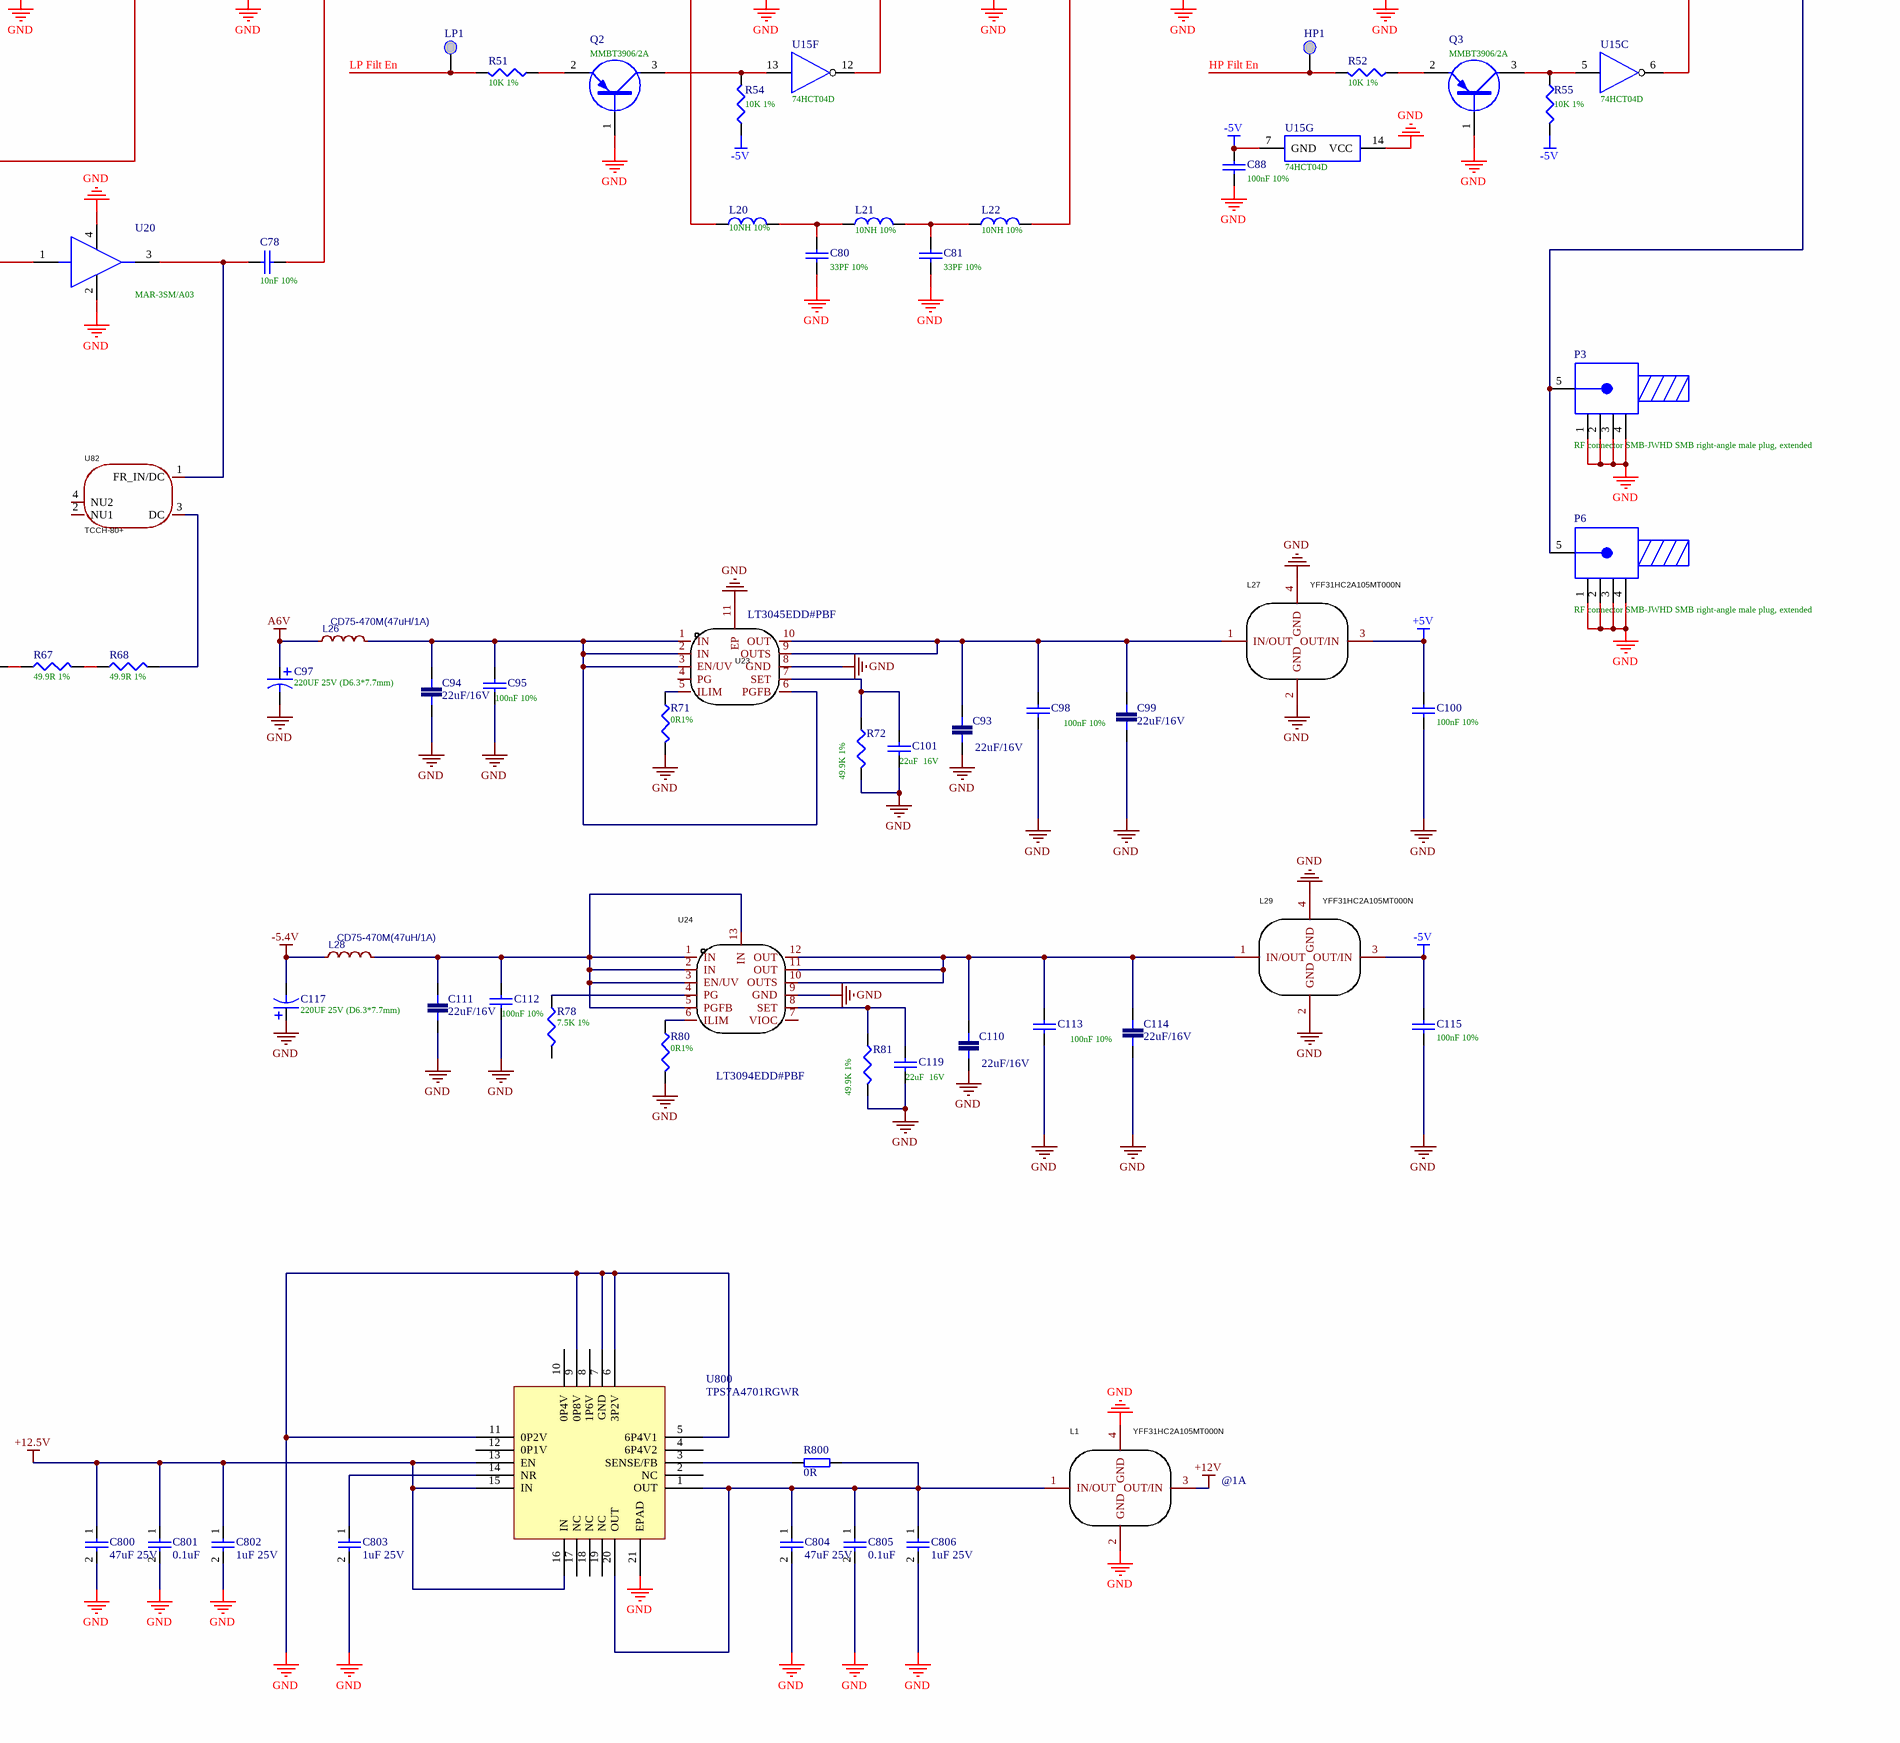
[diagram p0: PCBE109560-10.SchDoc, bottom right]
# Altium schematic sheet PCBE109560-10.SchDoc (part 2 of 2)

## Parts
1  (no value)  [DIP-1]
+1  (no value)  [DIP-1]
+2  (no value)  [DIP-1]
C4  20PF 10%  [0805C]
C5  330PF 10%  [1812C]
C6  22PF 10%  [1812C-2]
C7  22uF/16V  [0805]
C8  22uF/16V  [0805]
C9  100nF 10%  [0603]
C10  220UF 25V (D6.3*7.7mm)  [CAP-SMD_BD6.3-L6.6-W6.6-FD]
C11  100nF 10%  [0603]
C12  22uF/16V  [0805]
C13  100nF 10%  [0805R]
C14  22uF  16V  [0805]
C15  100nF 10%  [0805R]
C16  47PF 10%  [1812C-2]
C17  100PF 10%  [1812C-2]
C18  20PF 10%  [0805R]
C20  100nF 10%  [0805R]
C21  100nF 10%  [0805R]
C31  100nF 10%  [0805R]
C32  100nF 10%  [0805R]
C34  100nF 10%  [0805R]
C35  100nF 10%  [0805R]
C36  100nF 10%  [0805R]
C37  100nF 10%  [0805R]
C39  100nF 10%  [0805R]
C40  100nF 10%  [0805R]
C41  100nF 10%  [0805R]
C42  100nF 10%  [0805R]
C43  100nF 10%  [0805R]
C44  100nF 10%  [0805R]
C45  100nF 10%  [0805R]
C46  100nF 10%  [0805R]
C47  100nF 10%  [0805R]
C48  100nF 10%  [0805R]
C49  22uF 25V  [CAP-SMD_L6.0-W3.2-R-RD]
C50  100nF 10%  [0805R]
C51  100nF 10%  [0805R]
C52  100nF 10%  [0805R]
C53  3.3NF 10%  [0805R]
C54  100nF 10%  [0805R]
C55  330PF 10%  [0805R]
C56  330PF 10%  [0805R]
C57  100nF 10%  [0805R]
C58  33PF 10%  [0805R]
C59  33PF 10%  [0805R]
C60  100nF 10%  [0805R]
C61  100nF 10%  [0805R]
C62  100nF 10%  [0805R]
C63  100nF 10%  [0805R]
C64  100nF 10%  [0805R]
C65  33PF 10%  [0805R]
C66  33PF 10%  [0805R]
C67  100nF 10%  [0805R]
C68  39PF 10%  [0805R]
C69  100nF 10%  [0805R]
C70  25V 1UF Type A  [0805C-2]
C71  25V 1UF Type A  [0805C-2]
C72  100nF 10%  [0805R]
C73  25V 1UF Type A  [0805C-2]
C74  100nF 10%  [0805R]
C75  100nF 10%  [0805R]
C76  10nF 10%  [0805R]
C77  10nF 10%  [0805R]
C78  10nF 10%  [0805R]
C79  100nF 10%  [0603C]
C80  33PF 10%  [0805R]
C81  33PF 10%  [0805R]
C82  100nF 10%  [0805R]
C83  100nF 10%  [0805R]
C84  100nF 10%  [0805R]
C85  100nF 10%  [0805R]
C86  25V 1UF Type A  [0805C-2]
C87  3pF( ±0.1pF)  [0805R]
C88  100nF 10%  [0805R]
C89  100nF 10%  [0805R]
C90  100nF 10%  [0805R]
C93  22uF/16V  [0805]
C94  22uF/16V  [0805]
C95  100nF 10%  [0603]
C96  100nF 10%  [0805R]
C97  220UF 25V (D6.3*7.7mm)  [CAP-SMD_BD6.3-L6.6-W6.6-FD]
C98  100nF 10%  [0603]
C99  22uF/16V  [0805]
C100  100nF 10%  [0805R]
C101  22uF  16V  [0805]
C102  100nF 10%  [0805R]
C103  100nF 10%  [0805R]
C104  100nF 10%  [0805R]
C105  100nF 10%  [0805R]
C106  100nF 10%  [0805R]
C107  100nF 10%  [0805R]
C109  100nF 10%  [0805R]
C110  22uF/16V  [0805]
C111  22uF/16V  [0805]
C112  100nF 10%  [0603]
C113  100nF 10%  [0603]
C114  22uF/16V  [0805]
C115  100nF 10%  [0805R]
C116  100nF 10%  [0805R]
C117  220UF 25V (D6.3*7.7mm)  [CAP-SMD_BD6.3-L6.6-W6.6-FD]
C118  100nF 10%  [0805R]
C119  22uF  16V  [0805]
C122  100nF 10%  [0805R]
C123  100nF 10%  [0805R]
C124  100nF 10%  [0805R]
C125  100nF 10%  [0805R]
C128  100nF 10%  [0805R]
C129  100nF 10%  [0805R]
C130  100nF 10%  [0805R]
C800  47uF 25V  [1206]
C801  0.1uF  [0402]
C802  1uF 25V  [0402]
C803  1uF 25V  [0402]
C804  47uF 25V  [1206]
C805  0.1uF  [0402]
C806  1uF 25V  [0402]
C888  100nF 10%  [0805R]
Clk1  (no value)  [DIP-1]
D1  BAV99/A7  [SOT-23]
D2  GF1M-E3/67A/GM  [1808D]
D3  GF1M-E3/67A/GM  [1808D]
D4  GF1M-E3/67A/GM  [1808D]
D5  GF1M-E3/67A/GM  [1808D]
D8  BAV99/A7  [SOT-23-2]
D9  BAV99/A7  [SOT-23-2]
D10  BAV99/A7  [SOT-23-2]
D11  BAV99/A7  [SOT-23-2]
D12  BAV99/A7  [SOT-23-2]
Data1  (no value)  [DIP-1]
HP1  (no value)  [DIP-1]
J1  RF connector  [DIP-P]
J2  RF connector  [DIP-P]
L1  YFF31HC2A105MT000N  [FILTER-SMD_4P-L3.2-W1.6-L_YFF31HC]
L2  15UH 5%  [1005R]
L3  BLM21PG221SN1D(220Ω@100MHz)  [0805R]
L4  YFF31HC2A105MT000N  [FILTER-SMD_4P-L3.2-W1.6-L_YFF31HC]
L5  6.8UH 10%  [0805R]
L8  YFF31HC2A105MT000N  [FILTER-SMD_4P-L3.2-W1.6-L_YFF31HC]
L10  10NH 10%  [0805R]
L11  10NH 10%  [0805R]
L12  10NH 10%  [0805R]
L13  YFF31HC2A105MT000N  [FILTER-SMD_4P-L3.2-W1.6-L_YFF31HC]
L15  4.7UH 5%  [1005L]
L16  1UH 5%  [0805R]
L17  BLM21PG221SN1D(220Ω@100MHz)  [0805R]
L18  BLM21PG221SN1D(220Ω@100MHz  [0805R]
L19  NFM15PC104R1A3D  [FILTER-SMD_0402-3P-L1.0-W0.5-T]
L20  10NH 10%  [0805R]
L21  10NH 10%  [0805R]
L22  10NH 10%  [0805R]
L23  YFF31HC2A105MT000N  [FILTER-SMD_4P-L3.2-W1.6-L_YFF31HC]
L24  YFF31HC2A105MT000N  [FILTER-SMD_4P-L3.2-W1.6-L_YFF31HC]
L25  BLM21PG221SN1D(220Ω@100MHz  [0805R]
L26  CD75-470M(47uH/1A)  [IND-SMD_L7.8-W7.0-A]
L27  YFF31HC2A105MT000N  [FILTER-SMD_4P-L3.2-W1.6-L_YFF31HC]
L28  CD75-470M(47uH/1A)  [IND-SMD_L7.8-W7.0-A]
L29  YFF31HC2A105MT000N  [FILTER-SMD_4P-L3.2-W1.6-L_YFF31HC]
L31  BLM21PG221SN1D(220Ω@100MHz  [0805R]
L32  BLM21PG221SN1D(220Ω@100MHz  [0805R]
L808  NFM15PC104R1A3D  [FILTER-SMD_0402-3P-L1.0-W0.5-T]
L809  NFM15PC104R1A3D  [FILTER-SMD_0402-3P-L1.0-W0.5-T]
L810  NFM15PC104R1A3D  [FILTER-SMD_0402-3P-L1.0-W0.5-T]
L811  NFM15PC104R1A3D  [FILTER-SMD_0402-3P-L1.0-W0.5-T]
L812  NFM15PC104R1A3D  [FILTER-SMD_0402-3P-L1.0-W0.5-T]
L813  NFM15PC104R1A3D  [FILTER-SMD_0402-3P-L1.0-W0.5-T]
LP1  (no value)  [DIP-1]
P1  Header 20X2  [N0.8mm/40Pin-Plug]
P2  Header 4X2  [N0.8mm/8Pin-SOCKET]
P3  RF connector SMB-JWHD SMB right-angle male plug, extended  [DIP-P-2]
P4  Header 20X2  [N0.8mm/40Pin-Plug]
P5  Header 20X2  [N0.8mm/40Pin-Plug]
P6  RF connector SMB-JWHD SMB right-angle male plug, extended  [DIP-P-2]
Q1  MJD31C  [SOT-252-2]
Q2  MMBT3906/2A  [SOT-23]
Q3  MMBT3906/2A  [SOT-23]
Q4  MMBT3906/2A  [SOT-23]
R6  2K 5%  [0603R]
R7  NC  [AXIAL-0.51]
R8  3.9K 5% 1/2W  [AXIAL-0.51]
R9  3.9K 5% 1/2W  [AXIAL-0.51]
R10  3.9K 5% 1/2W  [AXIAL-0.51]
R11  3.9K 5% 1/2W  [AXIAL-0.51]
R13  0R1%  [0603]
R14  49.9K 1%  [0603]
R15  4.99K 1%  [0805R]
R16  2K 1%  [0805R]
R17  49.9R 1% 1/4W  [AXIAL-0.4]
R20  100R 1% 1/4W  [AXIAL-0.4]
R23  100R 1% 1/4W  [AXIAL-0.4]
R27  4.87K 1%  [0805R]
R28  4.87K 1%  [0805R]
R29  4.87K 1%  [0805R]
R30  4.87K 1%  [0805R]
R31  4.87K 1%  [0805R]
R32  10K 1%  [0805R]
R33  100K 1%  [0805R]
R34  100K 1%  [0805R]
R35  49.9R 1%  [0805R]
R36  49.9R 1%  [0805R]
R37  49.9R 1%  [0805R]
R38  49.9R 1%  [0805R]
R39  49.9R 1%  [0805R]
R40  49.9R 1% 1/4W  [R-SMD_L3.5-W1.5]
R41  10K 1%  [0805R]
R42  4.87K 1%  [0805R]
R43  4.87K 1%  [0805R]
R44  4.87K 1%  [0805R]
R45  4.87K 1%  [0805R]
R46  169R 1%  [0805R]
R47  169R 1%  [0805R]
R48  169R 1%  [0805R]
R49  49.9R 1%  [0805R]
R50  49.9R 1%  [0805R]
R51  10K 1%  [0805R]
R52  10K 1%  [0805R]
R53  10K 1%  [0805R]
R54  10K 1%  [0805R]
R55  10K 1%  [0805R]
R56  10K 1%  [0805R]
R57  10K 1%  [0805R]
R58  49.9R 1%  [0805R]
R59  4.99K 1%  [0805R]
R60  49.9R 1%  [R-SMD_L3.5-W1.5]
R61  30R 1%  [R-SMD_L3.5-W1.5]
R62  169R 1%  [0805R]
R63  169R 1%  [0805R]
R64  169R 1%  [0805R]
R65  49.9R 1%  [0805R]
R66  49.9R 1%  [0805R]
R67  49.9R 1%  [0805R]
R68  49.9R 1%  [0805R]
R69  120R 1%  [R-SMD_L3.5-W1.5]
R70  169R 1%  [0805R]
R71  0R1%  [0603]
R72  49.9K 1%  [0603]
R73  169R 1%  [0805R]
R74  NC  [0805R]
R75  169R 1%  [0805R]
R77  169R 1%  [0805R]
R78  7.5K 1%  [0603]
R80  0R1%  [0603]
R81  49.9K 1%  [0603]
R82  100K 1%  [0805R]
R83  10K 1%  [0805R]
R84  169R 1%  [0805R]
R800  0R  [0402]
RE1  AGQ210A4HZ  [RELAY-SMD_PANASONIC_AGQ2X0AXX]
RE2  AGQ210A4HZ  [RELAY-SMD_PANASONIC_AGQ2X0AXX]
RE3  AGQ210A4HZ  [RELAY-SMD_PANASONIC_AGQ2X0AXX]
RE4  AGQ210A4HZ  [RELAY-SMD_PANASONIC_AGQ2X0AXX]
RE5  AGQ210A4HZ  [RELAY-SMD_PANASONIC_AGQ2X0AXX]
Strobe1  (no value)  [DIP-1]
U4  LT3045EDD#PBF  [DFN-10_L3.0-W3.0-P0.50-BL-EP]
U6  74HCT123D  [SOIC-16_L9.9-W3.9-P1.27-LS6.0-BL]
U8  MAX504CSD+T  [SO-14]
U9  SW-239  [SO-8]
U11  SW-239  [SO-8]
U12  SW-239  [SO-8]
U13  SW-239  [SO-8]
U14  SW-239  [SO-8]
U15  74HCT04D  [SO-14]  (parts A,B,C,D,E,F,G of 7)
U16  AT-250(MAAV-007941)  [SO-8]
U17  MAR-3SM/A03  [LCC4]
U18  MAR-6SM/A06  [LCC4]
U19  MAR-6SM/A06  [LCC4]
U20  MAR-3SM/A03  [LCC4]
U21  MAX4106ESA+T  [SO-8]
U22  MIC4420CM  [SO-8]
U23  LT3045EDD#PBF  [DFN-10_L3.0-W3.0-P0.50-BL-EP]
U24  LT3094EDD#PBF  [WDFN-12_L3.0-W3.0-P0.45-BL-EP]
U25  AT65-0263  [SO-16]
U80  TCCH-80+  [IND-SMD_4P-L3.8-W3.8]
U81  TCCH-80+  [IND-SMD_4P-L3.8-W3.8]
U82  TCCH-80+  [IND-SMD_4P-L3.8-W3.8]
U83  TCCH-80+  [IND-SMD_4P-L3.8-W3.8]
U100  SW-239  [SO-8]
U800  TPS7A4701RGWR  [QFN-20]

## Nets
+5V: C100.1 C888.1 L25.1 L27.3(OUT/IN) L811.3(OUTPUT) L812.3(OUTPUT) U8.3(~{CLR})
+12.5V: +2.1 C106.1 C800.1 C801.1 C802.1 P5.31 P5.32 P5.33 P5.34 P5.35 P5.36 P5.37 P5.38 P5.39 P5.40 U800.13(EN) U800.15(IN) U800.16(IN)
+12V: C122.1 C123.1 C124.2 C125.2 L1.3(OUT/IN) L8.1(IN/OUT) L13.1(IN/OUT) U22.1(VS) U22.8(VS)
-5.4V: +1.1 C107.1 C117.2 L28.2 P5.1 P5.2 P5.3 P5.4 P5.5 P5.6 P5.7 P5.8 P5.9 P5.10
-5V: C88.2 C115.2 L29.3(OUT/IN) L809.1(INPUT) L810.3(OUTPUT) L813.3(OUTPUT) R54.1 R55.2 R57.1 U15.7(GND)
A6V: 1.1 C10.1 C97.1 C103.2 L3.1 L26.2 P5.17 P5.18 P5.19 P5.20 P5.21 P5.22 P5.23 P5.24
GND: C5.1 C6.2 C7.1 C8.1 C9.2 C10.2 C11.2 C12.1 C13.2 C14.2 C15.1 C18.2 C20.1 C21.1 C31.1 C32.1 C34.1 C35.1 C36.2 C37.2 C39.2 C40.2 C42.2 C43.1 C44.2 C45.2 C46.2 C47.1 C48.1 C49.2 C50.2 C57.2 C60.2 C61.1 C62.1 C63.1 C64.1 C65.2 C66.1 C70.1 C71.1 C72.2 C73.1 C74.1 C75.1 C80.1 C81.1 C83.2 C84.2 C85.1 C86.2 C88.1 C89.2 C90.2 C93.1 C94.1 C95.2 C96.2 C97.2 C98.2 C99.1 C100.2 C101.2 C102.2 C103.1 C104.2 C105.1 C106.2 C107.2 C109.2 C110.1 C111.1 C112.2 C113.2 C114.1 C115.1 C117.1 C118.2 C119.2 C122.2 C123.2 C124.1 C125.1 C128.1 C129.1 C130.2 C800.2 C801.2 C802.2 C803.2 C804.2 C805.2 C806.2 C888.2 D1.3 D2.2(K) D11.2 D12.1 J1.1 J1.2 J1.3 J1.4 J2.1 J2.2 J2.3 J2.4 L1.2(GND) L1.4(GND) L2.2 L4.2(GND) L4.4(GND) L8.2(GND) L8.4(GND) L13.2(GND) L13.4(GND) L15.2 L16.1 L19.2(GND) L23.2(GND) L23.4(GND) L24.2(GND) L24.4(GND) L27.2(GND) L27.4(GND) L29.2(GND) L29.4(GND) L808.2(GND) L809.2(GND) L810.2(GND) L811.2(GND) L812.2(GND) L813.2(GND) P1.5 P1.6 P1.11 P1.12 P1.17 P1.18 P1.20 P1.23 P1.24 P1.29 P1.30 P1.35 P1.36 P2.1 P2.3 P2.5 P2.7 P3.1 P3.2 P3.3 P3.4 P4.5 P4.6 P4.11 P4.12 P4.17 P4.18 P4.23 P4.24 P4.29 P4.30 P4.35 P4.36 P5.11 P5.12 P5.13 P5.14 P5.15 P5.16 P5.25 P5.26 P5.27 P5.28 P5.29 P5.30 P6.1 P6.2 P6.3 P6.4 Q1.2(E) Q2.1(B) Q3.1(B) Q4.1(B) R13.2 R14.2 R20.2 R32.2 R53.1 R59.1 R61.1 R71.2 R72.2 R74.1 R80.2 R81.2 R82.1 R83.1 RE1.3 RE3.6 RE4.2 U4.8(GND) U4.11(EP) U6.6(2CEXT) U6.8(GND) U6.10(2B) U6.14(1CEXT) U8.7(DGND) U8.8(AGND) U9.2(GND) U9.7(GND) U9.8(GND) U11.2(GND) U11.7(GND) U11.8(GND) U12.2(GND) U12.7(GND) U12.8(GND) U13.2(GND) U13.7(GND) U13.8(GND) U14.2(GND) U14.7(GND) U14.8(GND) U15.14(VCC) U16.2(GND) U16.3(GND) U16.5(GND) U16.6(GND) U16.7(GND) U17.2(GND) U17.4(GND) U18.2(GND) U18.4(GND) U19.2(GND) U19.4(GND) U20.2(GND) U20.4(GND) U22.4(GND) U22.5(GND) U23.8(GND) U23.11(EP) U24.9(GND) U25.2(GND) U25.3(GND) U25.4(GND) U25.5(GND) U25.6(GND) U25.7(GND) U25.16(GND) U100.2(GND) U100.7(GND) U100.8(GND) U800.5(6P4V1) U800.6(3P2V) U800.7(GND) U800.9(0P8V) U800.11(0P2V) U800.21(EPAD)
VCC: C13.1 C15.2 L4.3(OUT/IN) R15.1 R16.2 U6.2(1B) U6.3(1~{R}D) U6.16(VCC)
AK2: C21.2 P1.33 RE1.1
AK3: C20.2 P1.38 RE1.8
AK4: C37.1 P1.37 RE2.1
AK5: C36.1 P1.40 RE2.8
AK6: C31.2 P1.34 RE3.8
AK7: C32.2 P1.32 RE3.1
AK8: C34.2 C40.1 P1.28 RE4.8 RE5.8
AK9: C35.2 C39.1 P1.26 RE4.1 RE5.1
Attn1: P4.34 R70.2
Attn2: P4.32 R73.2
Attn4: P4.28 R75.2
Attn8: P4.26 R77.2
Attn16: P4.22 R84.2
DAC Clk: Clk1.1 P4.14 U8.4(SCLK)
DAC Data: Data1.1 P4.16 U8.2(DIN)
DAC Strobe: P4.10 Strobe1.1 U8.5(~{CS})
DATA_T: P1.39 R15.2 U6.1(1~{A})
HP Filt En: HP1.1 P4.4 R52.2
HT: L5.1 P2.2 P2.4 P2.6 P2.8
IN2: P4.8 R56.1 U22.2(IN)
LP Filt En: LP1.1 P4.2 R51.2
NetC4_1: C4.1 D1.2 L2.1 Q1.1(B) R6.1
NetC4_2: C4.2 R6.2 U6.13(1Q)
NetC5_2: C5.2 L5.2 R7.2
NetC6_1: C6.1 C16.2 C17.2 Q1.3(C) R11.1
NetC7_2: C7.2 C11.1 C12.2 L4.1(IN/OUT) U4.9(OUTS) U4.10(OUT)
NetC8_2: C8.2 C9.1 L3.2 U4.1(IN) U4.2(IN) U4.3(EN/UV) U4.6(PGFB)
NetC14_1: C14.1 R14.1 U4.7(SET)
NetC16_1: C16.1 D5.1(A) D8.2 D9.2 RE2.6
NetC17_1: C17.1 RE2.7
NetC18_1: C18.1 R16.1 U6.15(1REXT/CEXT)
NetC41_1: C41.1 U14.1(RFCOM)
NetC41_2: C41.2 P3.5 P6.5 R32.1
NetC42_1: C42.1 R27.1 U9.5(B)
NetC43_2: C43.2 R28.2 U100.4(A)
NetC44_1: C44.1 R29.1 U11.4(A)
NetC45_1: C45.1 R30.1 U12.5(B)
NetC46_1: C46.1 R31.1 U13.5(B) U14.4(A)
NetC47_2: C47.2 R35.1 U16.4(A)
NetC48_2: C48.2 L8.3(OUT/IN) R36.1
NetC49_1: C49.1 C50.1 U8.1(BIPOFF) U8.9(REFIN) U8.10(REFOUT)
NetC51_1: C51.1 U17.1(RF_IN)
NetC51_2: C51.2 U16.8(RF2)
NetC52_1: C52.1 L10.2
NetC52_2: C52.2 U17.3(RF_OUT) U81.1(FR_IN/DC)
NetC53_1: C53.1 C54.1 L15.1
NetC53_2: C53.2 U12.1(RFCOM)
NetC54_2: C54.2 U13.1(RFCOM)
NetC55_1: C55.1 U13.3(RF1)
NetC55_2: C55.2 C56.1 L16.2
NetC56_2: C56.2 U14.6(RF2)
NetC57_1: C57.1 R41.1 U13.4(A) U14.5(B)
NetC58_1: C58.1 C65.1
NetC58_2: C58.2 L10.1 L11.1
NetC59_1: C59.1 L11.2 L12.1
NetC59_2: C59.2 C66.2
NetC60_1: C60.1 R42.1 U9.4(A)
NetC61_2: C61.2 R43.2 U100.5(B)
NetC62_2: C62.2 R44.1 U11.5(B)
NetC63_2: C63.2 R45.1 U12.4(A)
NetC64_2: C64.2 L13.3(OUT/IN) R46.2
NetC67_1: C67.1 U18.1(RF_IN)
NetC67_2: C67.2 U25.1(RF)
NetC68_1: C68.1 C69.2 R49.2 R50.2
NetC68_2: C68.2 R49.1 R50.1 U18.3(RF_OUT) U80.1(FR_IN/DC)
NetC69_1: C69.1 R53.2 U16.1(RF1)
NetC70_2: C70.2 C74.2 L18.1 L19.1(INPUT)
NetC71_2: C71.2 C75.2 L19.3(OUTPUT) U21.4(VEE)
NetC72_1: C72.1 C73.2 L17.2 L18.2
NetC76_1: C76.1 U9.3(RF1)
NetC76_2: C76.2 U19.1(RF_IN)
NetC77_1: C77.1 U19.3(RF_OUT) U83.1(FR_IN/DC)
NetC77_2: C77.2 U20.1(RF_IN)
NetC78_1: C78.1 U20.3(RF_OUT) U82.1(FR_IN/DC)
NetC78_2: C78.2 U100.6(RF2)
NetC79_1: C79.1 D10.3 R40.2
NetC79_2: C79.2 R58.2 R59.2
NetC80_2: C80.2 L20.2 L21.2
NetC81_2: C81.2 L21.1 L22.1
NetC82_1: C82.1 R60.2
NetC82_2: C82.2 C116.1 R74.2 R82.2
NetC83_1: C83.1 C86.1 L808.1(INPUT) U21.7(VCC)
NetC84_1: C84.1 L23.3(OUT/IN) R62.2
NetC85_2: C85.2 L24.3(OUT/IN) R65.1
NetC87_1: C87.1 R60.1 R69.1 U21.6(OUT)
NetC87_2: C87.2 R61.2 R69.2 U21.2(IN-)
NetC89_1: C89.1 L813.1(INPUT) U8.11(VSS)
NetC90_1: C90.1 L32.2 L811.1(INPUT)
NetC93_2: C93.2 C98.1 C99.2 L27.1(IN/OUT) U23.9(OUTS) U23.10(OUT)
NetC94_2: C94.2 C95.1 L26.1 U23.1(IN) U23.2(IN) U23.3(EN/UV) U23.6(PGFB)
NetC96_1: C96.1 R70.1 U25.15(C1)
NetC101_1: C101.1 R72.1 U23.7(SET)
NetC102_1: C102.1 R73.1 U25.14(C2)
NetC104_1: C104.1 L812.1(INPUT) U8.13(VDD)
NetC105_2: C105.2 L31.1 L810.1(INPUT)
NetC109_1: C109.1 R75.1 U25.13(C4)
NetC110_2: C110.2 C113.1 C114.2 L29.1(IN/OUT) U24.10(OUTS) U24.11(OUT) U24.12(OUT)
NetC111_2: C111.2 C112.1 L28.1 U24.1(IN) U24.2(IN) U24.3(EN/UV) U24.5(PGFB) U24.13(IN)
NetC116_2: C116.2 R83.2 U25.8(RF)
NetC118_1: C118.1 R77.1 U25.12(C8)
NetC119_1: C119.1 R81.1 U24.8(SET)
NetC128_2: C128.2 L31.2 U25.11(VEE)
NetC129_2: C129.2 L32.1 U25.10(VCC)
NetC130_1: C130.1 R84.1 U25.9(C16)
NetC803_1: C803.1 U800.14(NR)
NetC804_1: C804.1 C805.1 C806.1 L1.1(IN/OUT) R800.1 U800.1(OUT) U800.20(OUT)
NetD2_1: D2.1(A) D3.2(K)
NetD3_1: D3.1(A) D4.2(K)
NetD4_1: D4.1(A) D5.2(K)
NetD8_1: D8.1 D9.1 J1.5 R17.1 R20.1 R23.1 RE4.4
NetD10_1: D10.1 D12.2
NetD10_2: D10.2 D11.1
NetJ2_5: J2.5 RE5.4
NetL12_2: L12.2 U9.1(RFCOM)
NetL17_1: L17.1 L809.3(OUTPUT)
NetL20_1: L20.1 U11.6(RF2)
NetL22_2: L22.2 U12.3(RF1)
NetL23_1: L23.1(IN/OUT) L24.1(IN/OUT) U22.6(OUT) U22.7(OUT)
NetL25_2: L25.2 L808.3(OUTPUT)
NetQ2_2: Q2.2(E) R51.1
NetQ2_3: Q2.3(C) R54.2 U15.13(6A)
NetQ3_2: Q3.2(E) R52.1
NetQ3_3: Q3.3(C) R55.1 U15.5(3A)
NetQ4_2: Q4.2(E) R56.2
NetQ4_3: Q4.3(C) R57.2 U15.1(1A)
NetR7_1: R7.1 R8.1
NetR8_2: R8.2 R9.2
NetR9_1: R9.1 R10.1
NetR10_2: R10.2 R11.2
NetR13_1: R13.1 U4.5(ILIM)
NetR17_2: R17.2 RE1.2
NetR23_2: R23.2 RE3.7
NetR27_2: R27.2 R28.1 U15.4(2Y)
NetR29_2: R29.2 R30.2 U15.10(5Y)
NetR31_2: R31.2 U15.8(4Y)
NetR33_1: R33.1 R34.1 U8.14(RFB)
NetR33_2: R33.2 R34.2 R35.2 U8.12(VOUT)
NetR36_2: R36.2 R37.1
NetR37_2: R37.2 R38.2
NetR38_1: R38.1 R39.1
NetR39_2: R39.2 U81.3(DC)
NetR40_1: R40.1 RE5.3
NetR41_2: R41.2 U15.6(3Y) U15.9(4A)
NetR42_2: R42.2 R43.1 U15.2(1Y) U15.3(2A)
NetR44_2: R44.2 R45.2 U15.11(5A) U15.12(6Y)
NetR46_1: R46.1 R47.2
NetR47_1: R47.1 R48.1
NetR48_2: R48.2 U80.3(DC)
NetR58_1: R58.1 U21.3(IN+)
NetR62_1: R62.1 R63.1
NetR63_2: R63.2 R64.2
NetR64_1: R64.1 U83.3(DC)
NetR65_2: R65.2 R66.2
NetR66_1: R66.1 R67.1
NetR67_2: R67.2 R68.1
NetR68_2: R68.2 U82.3(DC)
NetR71_1: R71.1 U23.5(ILIM)
NetR78_1: R78.1 U24.4(PG)
NetR80_1: R80.1 U24.6(ILIM)
NetR800_2: R800.2 U800.3(SENSE/FB)
NetRE4_3: RE4.3 RE5.2
NetU9_6: U9.6(RF2) U100.3(RF1)
NetU11_1: U11.1(RFCOM) U100.1(RFCOM)
NetU11_3: U11.3(RF1) U12.6(RF2)
NetU13_6: U13.6(RF2) U14.3(RF1)

Not connected (* = marked no-connect by the designer): D1 1*; D8 3; D9 3; D11 3; D12 3; P1 1 2 3 4 7 8 9 10 13 14 15 16 19 21 22 25 27 31; P4 1 3 7 9 13 15 19 20 21 25 27 31 33 37 38 39 40; R78 2; RE1 4 5 6 7; RE2 2 3 4 5; RE3 2 3 4 5; RE4 5 6 7; RE5 5 6 7; U4 4(PG); U6 4(1~{Q}) 5(2Q) 7(2REXT/CEXT) 9(2~{A}) 11(2~{R}D) 12(2~{Q}); U8 6(DOUT); U22 3(NC); U23 4(PG); U24 7(VIOC); U80 2(NU1) 4(NU2); U81 2(NU1) 4(NU2); U82 2(NU1) 4(NU2); U83 2(NU1) 4(NU2); U800 2(NC) 4(6P4V2) 8(1P6V) 10(0P4V) 12(0P1V) 17(NC) 18(NC) 19(NC)

## Notes on the sheet
- (near P1) Transmit interface
- 500V high-voltage interface
- Receive interface
- @1A

## Library data of the parts
1 +1 +2 Clk1 Data1 HP1 LP1 Strobe1 = TP
C4-C6 C9 C11 C13-C18 C20 C21 C31 C32 C34-C37 C39-C48 C50-C69 C72-C85 C87-C90 C95 C96 C98 C100-C107 C109 C112 C113 C115 C116 C118 C119 C122-C125 C128-C130 C800-C806 C888 = CAP: Capacitor
C7 C8 C12 C93 C94 C99 C110 C111 C114 = C1206
C10 C97 C117 = CAPACITOR_1: Capacitor
C49 = TAJC226K025RNJ: Manufacturer: Kyocera AVX; Add into BOM: yes; Tolerance: ±10%; Equivalent Series Resistance(ESR): 1.4Ω@100kHz; Symbol: TAJC226K025RNJ; Device: TAJC226K025RNJ; LCSC Part Name: 22uF ±10% 25V; Supplier Part: C7214; Manufacturer Part: TAJC226K025RNJ; Supplier Footprint: CASE-C-6032; JLCPCB Part Class: Extended Part; Datasheet: https://atta.szlcsc.com/upload/public/pdf/source/20160107/1457707750344.pdf; Supplier: LCSC; Convert to PCB: yes; Value: 22uF; Rated Voltage: 25V; Operating Temperature: -55℃~+125℃
C70 C71 C86 = CAPACITOR POL: Capacitor
D1 D8-D12 = BAV99
D2-D5 = DIODE
J1 J2 = SMA-KWE: BOM_Supplier: *; BOM_Supplier Part: *; BOM_Manufacturer: *; BOM_Manufacturer Part: *; BOM_JLCPCB Part Class: *; spicePre: *; spiceSymbolName: *; Contributor: *
L1 L4 L8 L13 L23 L24 L27 L29 = YFF31HC2A105MT000N: Manufacturer: TDK; Add into BOM: yes; Nominal Capacitance: 1uF; CapacitanceTolerance: ±20%; DC Rated Voltage: 100V; Rated Current: 6A; DC Resistance: 5mΩ; Name: YFF31HC2A105MT000N; Symbol: YFF31HC2A105MT000N; Device: YFF31HC2A105MT000N; LCSC Part Name: 1uF(105) ±20% 100V; Supplier Part: C113216; Manufacturer Part: YFF31HC2A105MT000N; Supplier Footprint: SMD-4P,1.6x3.2mm; JLCPCB Part Class: Extended Part; Datasheet: https://atta.szlcsc.com/upload/public/pdf/source/20180326/C113216_F6F81E50B9805DA3D7C436129903DEBD.pdf; Supplier: LCSC; Convert to PCB: yes; Operating Temperature: -55℃~+125℃
L2 L3 L5 L10-L12 L15-L18 L20-L22 L25 L31 L32 = INDUCTOR
L19 L808-L813 = NFM15PC104R1A3D: Manufacturer: muRata(村田); Add into BOM: yes; Nominal Capacitance: 100nF; CapacitanceTolerance: ±20%; DC Rated Voltage: 10V; Rated Current: 2A; DC Resistance: 30mΩ; Symbol: NFM15PC104R1A3D; Device: NFM15PC104R1A3D; LCSC Part Name: 0.1uF ±20% 10V; Supplier Part: C2650905; Manufacturer Part: NFM15PC104R1A3D; Supplier Footprint: 0402; JLCPCB Part Class: Extended Part; Datasheet: https://atta.szlcsc.com/upload/public/pdf/source/20210611/05FD8D968916F804F398094FB2B4AAFE.pdf; Supplier: LCSC; Convert to PCB: yes; Operating Temperature: -55℃~+105℃; Comment_1: NFM15PC104R1A3D
L26 L28 = 4.7uH/5a: BOM_Manufacturer: COILMX; BOM_Manufacturer Part: MS0630-4R7M; nameAlias: Inductance; Contributor: LCSC; BOM_Supplier: LCSC; BOM_Supplier Part: C380177; spicePre: L; spiceSymbolName: MS0630-4R7M
P1 P4 P5 = Header 20X2: Header, 20-Pin, Dual row; LatestRevisionDate: 17-Jul-2002; LatestRevisionNote: Re-released for DXP Platform.; Publisher: Altium Limited
P2 = Header 4X2: Header, 4-Pin, Dual row; LatestRevisionDate: 17-Jul-2002; LatestRevisionNote: Re-released for DXP Platform.; Publisher: Altium Limited
P3 P6 = JA1
Q1 = NPN: NPN Transistor
Q2-Q4 = PNP: PNP Transistor
R6-R11 R13-R17 R20 R23 R27-R75 R77 R78 R80-R84 = RES1
R800 = RES
RE1-RE5 = AGQ210A4HZ: Manufacturer: PANASONIC(松下); Add into BOM: yes; Coil Voltage: 4.5V; Contact Form: Two changeover sets: 2C (DPDT changeover); Maximum Switching Voltage: 125V@AC; 110V@DC; Coil Type: Single coil; Maximum Switching Current: 2A; Operate Time: 4ms; Symbol: AGQ210A4HZ; Device: AGQ210A4HZ; LCSC Part Name: AGQ210A4HZ; Supplier Part: C2153577; Manufacturer Part: AGQ210A4HZ; Supplier Footprint: SMD,7.2x10.6mm; JLCPCB Part Class: Extended Part; Datasheet: https://atta.szlcsc.com/upload/public/pdf/source/20210727/C2858037_82AE1FE69E1888D41D6E9B5D42950540.pdf; Supplier: LCSC; Convert to PCB: yes; Pin Number: -; Contact Rating: -; Contact Material: AgPd + gold plating; Coil Rated Power: -; Coil Resistance: -; Release Time: 4ms; Contact Resistance: -; Operating Temperature: -40℃~+85℃; Comment_1: AGQ210A4HZ
U4 U23 = LT3045EDD#PBF: Symbol: LT3045EDD#PBF_C666574; Add into BOM: yes; Maximum Input Voltage: 20V; Output Voltage: 0V~15V; MAX Output Current: 500mA; Dropout Voltage: 450mV@(500mA); standby current: 20uA; Number of Outputs: 1; Device: LT3045EDD#PBF; LCSC Part Name: LT3045EDD#PBF; Supplier Part: C666574; Manufacturer Part: LT3045EDD#PBF; Supplier Footprint: DFN-10-EP(3x3); JLCPCB Part Class: Extended Part; Datasheet: https://atta.szlcsc.com/upload/public/pdf/source/20200416/C514420_E440C492D6C74EAE6AB301243586F696.pdf; Supplier: LCSC; Convert to PCB: yes
U15 = 74HC04
U16 = AT-250
U17 U20 = MAR-3SM
U18 U19 = MAR-6SM
U21 = MAX4107ESA: Manufacturer: *; Manufacturer Part: *; Supplier Part: *; Supplier: *; link: *; spicePre: *; spiceSymbolName: *; Package Display: *; Contributor: *
U24 = LT3094EDD#PBF: Add into BOM: yes; Symbol: LT3094EDD#PBF; Device: LT3094EDD#PBF; LCSC Part Name: LT3094EDD#PBF; Supplier Part: C670492; Manufacturer Part: LT3094EDD#PBF; Supplier Footprint: WDFN-12-EP(3x3); JLCPCB Part Class: Extended Part; Datasheet: https://atta.szlcsc.com/upload/public/pdf/source/20200318/C498217_A5485280C797CF3891C55BEBE66C21D4.pdf; Supplier: LCSC; Convert to PCB: yes; Output Type: -
U80-U83 = TCCH-80+: Manufacturer: Mini-Circuits; Add into BOM: yes; Value: 4uH; Rated Current: 200mA; DC Resistance (DCR): 100mΩ; Symbol: TCCH-80+; Device: TCCH-80+; LCSC Part Name: 4uH; Supplier Part: C3223029; Manufacturer Part: TCCH-80+; Supplier Footprint: SMD-4P,3.8x3.8mm; JLCPCB Part Class: Extended Part; Datasheet: https://atta.szlcsc.com/upload/public/pdf/source/20240402/75EC49D4FFFA61CBEC009CC2CCA83C83.pdf; Supplier: LCSC; Convert to PCB: yes; Tolerance: -; Saturation Current (Isat): -; Type: -; Ratings: -
U800 = TPS7A4701RGWR(QFN20): Name: *; Symbol: *; Device: *; LCSC Part Name: *; Supplier Part: *; Manufacturer: *; Manufacturer Part: *; Supplier Footprint: *; JLCPCB Part Class: *; Datasheet: *; Supplier: *; Add into BOM: *; Convert to PCB: *; Output Type: *; Output Polarity: *; Number of Outputs: *